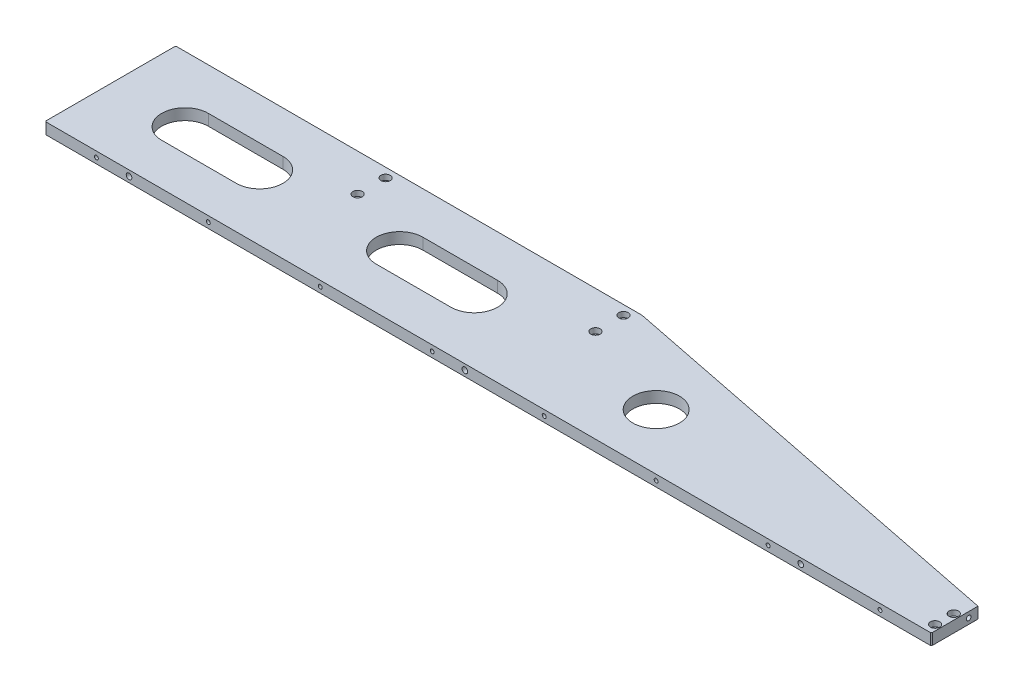
SolidWorks part; units mm, degrees
material "A7075"
ref_plane "Front Plane" through (0, 0, 0) normal (0, 0, 1) x (1, 0, 0)
ref_plane "Top Plane" through (0, 0, 0) normal (0, 1, 0) x (1, 0, 0)
ref_plane "Right Plane" through (0, 0, 0) normal (1, 0, 0) x (0, 0, -1)
sketch "Sketch2" plane through (0, 0, 0) normal (0, -1, 0) x (-1, 0, 0)
  line L0 (0, 0) -> (0, 140)
  line L1 (0, 140) -> (-500, 140)
  line L2 (-500, 140) -> (-950, 50)
  line L3 (-950, 50) -> (-950, 0)
  line L6 (0, 0) -> (-950, 0)
  dimension "D1" = 950
  dimension "D2" = 500
  dimension "D3" = 50
  dimension "D4" = 140
extrude "Boss-Extrude2" add sketch "Sketch2" against normal blind 12 separate body
sketch "Sketch9" plane through (0, 0, 0) normal (0, -1, 0) x (1, 0, 0)
  line L0 (80, -70) -> (160, -70) construction
  line L1 (80, -45) -> (160, -45)
  line L2 (80, -95) -> (160, -95)
  line L3 (310, -70) -> (390, -70) construction
  line L4 (310, -45) -> (390, -45)
  line L5 (310, -95) -> (390, -95)
  line L14 (950, 0) -> (0, 0) construction
  line L15 (0, 0) -> (0, -140) construction
  arc A0 (80, -45) -> (80, -95) centre (80, -70) ccw
  arc A1 (160, -95) -> (160, -45) centre (160, -70) ccw
  arc A2 (310, -45) -> (310, -95) centre (310, -70) ccw
  arc A3 (390, -95) -> (390, -45) centre (390, -70) ccw
  circle A4 centre (595, -60) radius 25
  point P2 (120, -70)
  point P7 (350, -70)
  dimension "D3" = 150
  dimension "D4" = 70
  dimension "D5" = 80
  dimension "D6" = 50
  dimension "D7" = 60
  dimension "D8" = 595
  dimension "D1" = 50
  dimension "D2" = 80
extrude "Cut-Extrude3" cut sketch "Sketch9" against normal blind 12
hole_wizard "M4 Tapped Hole3" positions "Sketch25" profile "Sketch24" tap size "M4" standard "Gb"
sketch "Sketch25" plane through (0, 0, -140) normal (0, 0, -1) x (-1, 0, 0)
  line L1 (0, 0) -> (-500, 0) construction
  line L2 (0, 12) -> (0, 0) construction
  point P0 (-50, 6)
  point P4 (-400, 6)
  dimension "D1" = 50
  dimension "D2" = 350
  dimension "D4" = 6
sketch "Sketch24" plane through (50, 6, -140) normal (1, 0, 0) x (0, 1, 0)
  line L0 (0, 0) -> (0, 12.4914)
  line L1 (0, 12.4914) -> (1.65, 11.5)
  line L2 (1.65, 11.5) -> (1.65, 0)
  line L5 (1.65, 0) -> (0, 0)
  line L10 (0, 12.4914) -> (-1.65, 11.5) construction
  line L11 (0, -6.35) -> (0, 107.95) construction
  dimension "螺纹孔钻头直径" = 3.3
  dimension "螺纹孔钻头深度" = 11.5
  dimension "导头角度" = 118
cosmetic thread "Cosmetic thread 15" parameters "D1"=8, "D2"=4
cosmetic thread "Cosmetic thread 17" parameters "D1"=8, "D2"=4
hole_wizard "M4 Tapped Hole4" positions "Sketch27" profile "Sketch26" tap size "M4" standard "Gb"
sketch "Sketch27" plane through (46.1538, 0, -230.7692) normal (0.1961, 0, -0.9806) x (-0.9806, 0, -0.1961)
  line L0 (-462.8341, 0) -> (-921.7458, 0) construction
  line L2 (-921.7458, 12) -> (-921.7458, 0) construction
  point P4 (-871.7458, 6)
  point P6 (-521.7458, 6)
  dimension "D1" = 50
  dimension "D2" = 350
  dimension "D3" = 6
sketch "Sketch26" plane through (900.971, 6, -59.8058) normal (0, 1, 0) x (-0.9806, 0, -0.1961)
  line L0 (0, 0) -> (0, 12.4914)
  line L1 (0, 12.4914) -> (1.65, 11.5)
  line L2 (1.65, 11.5) -> (1.65, 0)
  line L5 (1.65, 0) -> (0, 0)
  line L10 (0, 12.4914) -> (-1.65, 11.5) construction
  line L11 (0, -6.35) -> (0, 107.95) construction
  dimension "螺纹孔钻头直径" = 3.3
  dimension "螺纹孔钻头深度" = 11.5
  dimension "导头角度" = 118
cosmetic thread "Cosmetic thread 18" parameters "D1"=8, "D2"=4
cosmetic thread "Cosmetic thread 19" parameters "D1"=8, "D2"=4
hole_wizard "M6 Tapped Hole3" positions "Sketch29" profile "Sketch28" tap size "M6" standard "Gb"
sketch "Sketch29" plane through (950, 0, 0) normal (1, 0, 0) x (0, 0, -1)
  line L0 (50, 0) -> (0, 0) construction
  line L1 (50, 12) -> (50, 0) construction
  point P0 (40, 6)
  point P2 (40, 96)
  dimension "D1" = 90
  dimension "D2" = 6
  dimension "D3" = 10
sketch "Sketch28" plane through (950, 6, -40) normal (0, 1, 0) x (0, 0, -1)
  line L0 (0, 0) -> (0, 18.5022)
  line L1 (0, 18.5022) -> (2.5, 17)
  line L2 (2.5, 17) -> (2.5, 0)
  line L5 (2.5, 0) -> (0, 0)
  line L10 (0, 18.5022) -> (-2.5, 17) construction
  line L11 (0, -6.35) -> (0, 107.95) construction
  dimension "螺纹孔钻头直径" = 5
  dimension "螺纹孔钻头深度" = 17
  dimension "导头角度" = 118
cosmetic thread "Cosmetic thread 23" parameters "D1"=12, "D2"=6
hole_wizard "M6 Tapped Hole2" positions "Sketch31" profile "Sketch30" tap size "M6" standard "Iso"
sketch "Sketch31" plane through (0, 0, 0) normal (-1, 0, 0) x (0, 0, 1)
  line L0 (-15, 6) -> (0, 6) construction
  line L1 (0, 12) -> (0, 0) construction
  point P0 (-15, 6)
  point P2 (-70, 6)
  point P4 (-125, 6)
  dimension "D1" = 110
  dimension "D2" = 15
  dimension "D3" = 55
sketch "Sketch30" plane through (0, 6, -15) normal (0, 1, 0) x (0, 0, 1)
  line L0 (0, 0) -> (0, 24.5022)
  line L1 (0, 24.5022) -> (2.5, 23)
  line L2 (2.5, 23) -> (2.5, 0)
  line L5 (2.5, 0) -> (0, 0)
  line L10 (0, 24.5022) -> (-2.5, 23) construction
  line L11 (0, -6.35) -> (0, 107.95) construction
  dimension "螺纹孔钻头直径" = 5
  dimension "螺纹孔钻头深度" = 23
  dimension "导头角度" = 118
cosmetic thread "Cosmetic thread 25" parameters "D1"=20, "D2"=6
cosmetic thread "Cosmetic thread 26" parameters "D1"=20, "D2"=6
cosmetic thread "Cosmetic thread 27" parameters "D1"=20, "D2"=6
hole_wizard "Ø6.0 (6) Diameter Hole1" positions "Sketch33" profile "Sketch32" hole size "Ø6.0" standard "Gb"
sketch "Sketch33" plane through (0, 0, 0) normal (-1, 0, 0) x (0, 0, 1)
  line L1 (0, 12) -> (0, 0) construction
  circle A0 centre (-70, 6) radius 2.5 construction
  point P0 (-30, 6)
  point P2 (-110, 6)
  point P9 (0, 6)
  dimension "D1" = 80
  dimension "D2" = 40
sketch "Sketch32" plane through (0, 6, -30) normal (0, 1, 0) x (0, 0, 1)
  line L0 (0, 0) -> (0, 16.8026)
  line L1 (0, 16.8026) -> (3, 15)
  line L2 (3, 15) -> (3, 0)
  line L5 (3, 0) -> (0, 0)
  line L10 (0, 16.8026) -> (-3, 15) construction
  line L11 (0, -6.35) -> (0, 107.95) construction
  dimension "孔直径" = 6
  dimension "孔深度" = 15
  dimension "导头角度" = 118
hole_wizard "M5 Tapped Hole1" positions "Sketch36" profile "Sketch34" tap size "M5" standard "Iso"
sketch "Sketch36" plane through (0, 0, 0) normal (0, 0, 1) x (1, 0, 0)
  line L0 (0, 6) -> (1106.8343, 6) construction
  line L1 (0, 12) -> (0, 0) construction
  point P0 (55, 6)
  point P10 (175, 6)
  point P12 (295, 6)
  point P14 (415, 6)
  point P16 (535, 6)
  point P18 (655, 6)
  point P20 (775, 6)
  point P22 (895, 6)
  dimension "D3" = 120
  dimension "D4" = 120
  dimension "D5" = 120
  dimension "D6" = 120
  dimension "D7" = 120
  dimension "D8" = 120
  dimension "D9" = 120
  dimension "D10" = 55
sketch "Sketch34" plane through (55, 6, 0) normal (1, 0, 0) x (0, -1, 0)
  line L0 (0, 0) -> (0, 13.6618)
  line L1 (0, 13.6618) -> (2.1, 12.4)
  line L2 (2.1, 12.4) -> (2.1, 0)
  line L5 (2.1, 0) -> (0, 0)
  line L10 (0, 13.6618) -> (-2.1, 12.4) construction
  line L11 (0, -6.35) -> (0, 107.95) construction
  dimension "螺纹孔钻头直径" = 4.2
  dimension "螺纹孔钻头深度" = 12.4
  dimension "导头角度" = 118
cosmetic thread "Cosmetic thread 30" parameters "D1"=10, "D2"=5
cosmetic thread "Cosmetic thread 31" parameters "D1"=10, "D2"=5
cosmetic thread "Cosmetic thread 32" parameters "D1"=10, "D2"=5
cosmetic thread "Cosmetic thread 33" parameters "D1"=10, "D2"=5
cosmetic thread "Cosmetic thread 34" parameters "D1"=10, "D2"=5
cosmetic thread "Cosmetic thread 35" parameters "D1"=10, "D2"=5
cosmetic thread "Cosmetic thread 36" parameters "D1"=10, "D2"=5
cosmetic thread "Cosmetic thread 37" parameters "D1"=10, "D2"=5
hole_wizard "Ø6.0 (6) Diameter Hole2" positions "Sketch38" profile "Sketch37" hole size "Ø6.0" standard "Gb"
sketch "Sketch38" plane through (0, 0, 0) normal (0, 0, 1) x (1, 0, 0)
  line L0 (0, 12) -> (0, 0) construction
  point P0 (90, 6)
  point P2 (450, 6)
  point P4 (810, 6)
  point P13 (0, 6)
  dimension "D1" = 90
  dimension "D2" = 360
  dimension "D3" = 360
sketch "Sketch37" plane through (90, 6, 0) normal (1, 0, 0) x (0, -1, 0)
  line L0 (0, 0) -> (0, 16.8026)
  line L1 (0, 16.8026) -> (3, 15)
  line L2 (3, 15) -> (3, 0)
  line L5 (3, 0) -> (0, 0)
  line L10 (0, 16.8026) -> (-3, 15) construction
  line L11 (0, -6.35) -> (0, 107.95) construction
  dimension "孔直径" = 6
  dimension "孔深度" = 15
  dimension "导头角度" = 118
hole_wizard "Hole size per hex socket screw type1" positions "Sketch40" profile "Sketch39" counterbore size "M5" standard "Gb" end condition through all
sketch "Sketch40" plane through (-526.9587, 12, -55.4794) normal (0, -1, 0) x (-1, 0, 0)
  line L0 (-526.9587, 84.5206) -> (-1026.9587, 84.5206) construction
  line L1 (-526.9587, -55.4794) -> (-526.9587, 84.5206) construction
  line L2 (-1476.9587, -5.4794) -> (-1476.9587, -55.4794) construction
  line L3 (-1476.9587, -55.4794) -> (-526.9587, -55.4794) construction
  point P0 (-761.9587, 44.5206)
  point P2 (-761.9587, 74.5206)
  point P4 (-1016.9587, 44.5206)
  point P6 (-1016.9587, 74.5206)
  point P8 (-1470.9587, -45.4794)
  point P10 (-1470.9587, -25.4794)
  dimension "D1" = 30
  dimension "D2" = 10
  dimension "D3" = 235
  dimension "D4" = 255
  dimension "D5" = 6
  dimension "D6" = 10
  dimension "D7" = 20
sketch "Sketch39" plane through (235, 12, -100) normal (1, 0, 0) x (0, 0, 1)
  line L0 (0, 0) -> (0, 12)
  line L1 (0, 12) -> (2.75, 12)
  line L3 (2.75, 12) -> (2.75, 5.7)
  line L4 (2.75, 5.7) -> (5, 5.7)
  line L5 (5, 5.7) -> (5, 0)
  line L7 (5, 0) -> (0, 0)
  line L11 (0, -6.35) -> (0, 107.95) construction
  dimension "通孔孔直径" = 5.5
  dimension "通孔孔深度" = 12
  dimension "柱形沉头孔直径" = 10
  dimension "柱形沉头孔深度" = 5.7
chamfer "Chamfer1" distance 1 angle 45 3 edges at (0, 6, -140) (0, 6, 0) (950, 6, 0)
